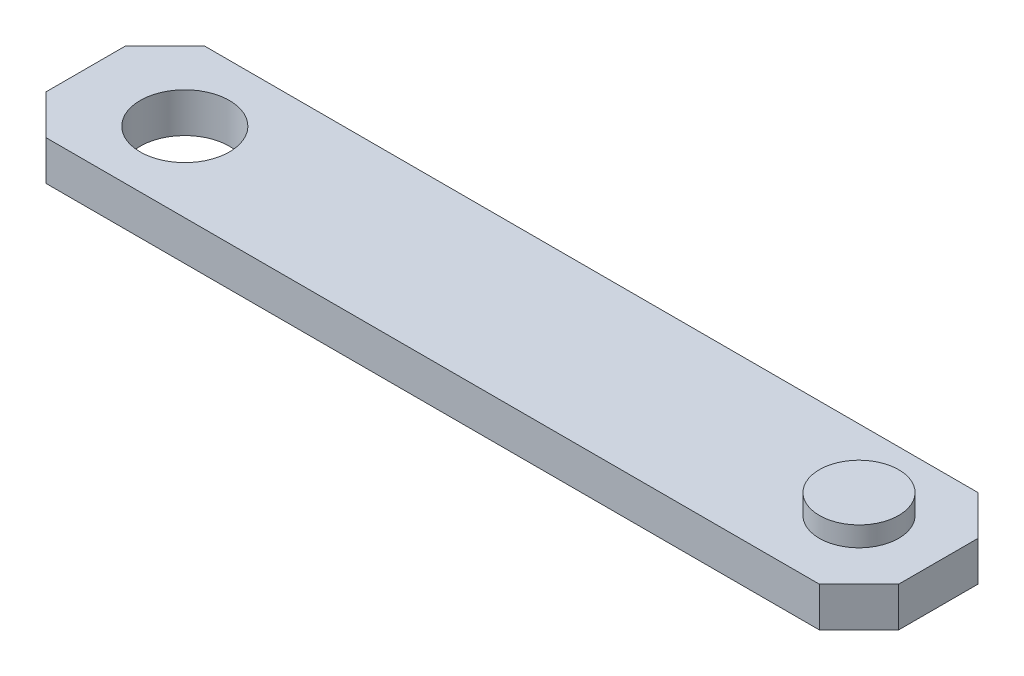
SolidWorks part; units mm, degrees
ref_plane "Front Plane" through (0, 0, 0) normal (0, 0, 1) x (1, 0, 0)
ref_plane "Top Plane" through (0, 0, 0) normal (0, 1, 0) x (1, 0, 0)
ref_plane "Right Plane" through (0, 0, 0) normal (1, 0, 0) x (0, 0, -1)
sketch "Sketch1" plane through (0, 0, 0) normal (0, 1, 0) x (1, 0, 0)
  line L1 (-9.6934, 7.4844) -> (33.3066, 7.4844)
  line L2 (-9.6934, 7.4844) -> (-9.6934, -0.5156)
  line L3 (-9.6934, -0.5156) -> (33.3066, -0.5156)
  line L4 (33.3066, 7.4844) -> (33.3066, -0.5156)
  dimension "D1" = 43
  dimension "D2" = 8
extrude "Boss-Extrude1" add sketch "Sketch1" along normal blind 2
sketch "Sketch2" plane through (0, 2, 0) normal (0, 1, 0) x (1, 0, 0)
  line L0 (33.3066, 7.4844) -> (-9.6934, 7.4844) construction
  line L1 (-9.6934, 7.4844) -> (-9.6934, -0.5156) construction
  circle A0 centre (-4.6934, 3.4844) radius 2.25
  dimension "D3" = 4.5
  dimension "D1" = 4
  dimension "D2" = 5
extrude "Cut-Extrude1" cut sketch "Sketch2" against normal through all
sketch "Sketch3" plane through (0, 2, 0) normal (0, 1, 0) x (1, 0, 0)
  line L0 (33.3066, 7.4844) -> (-9.6934, 7.4844) construction
  line L1 (33.3066, -0.5156) -> (33.3066, 7.4844) construction
  circle A0 centre (29.3066, 3.4844) radius 2
  dimension "D2" = 4
  dimension "D3" = 4
  dimension "D1" = 4
extrude "Boss-Extrude2" add sketch "Sketch3" along normal blind 1
chamfer "Chamfer1" [suppressed] distance 0.5 angle 45
chamfer "Chamfer2" distance 2 angle 45 4 edges at (33.3066, 1, -7.4844) (33.3066, 1, 0.5156) (-9.6934, 1, -7.4844) (-9.6934, 1, 0.5156)
